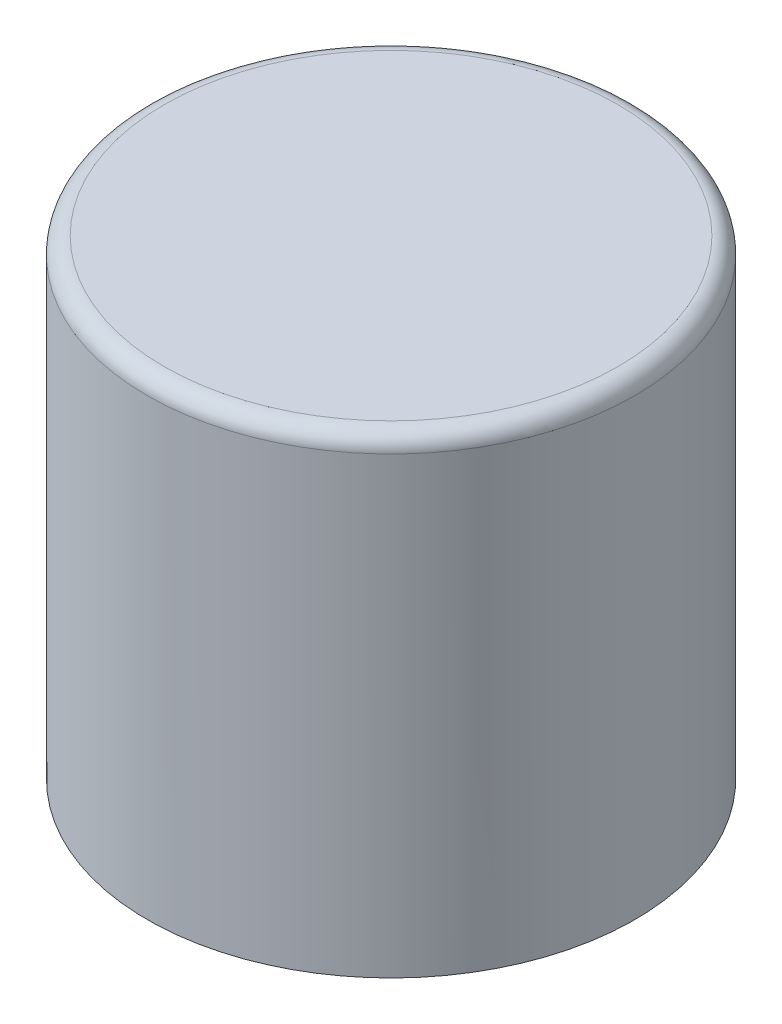
SolidWorks part; units mm, degrees
ref_plane "前视基准面" through (0, 0, 0) normal (0, 0, 1) x (1, 0, 0)
ref_plane "上视基准面" through (0, 0, 0) normal (0, 1, 0) x (1, 0, 0)
ref_plane "右视基准面" through (0, 0, 0) normal (1, 0, 0) x (0, 0, -1)
sketch "草图1" plane through (0, 0, 0) normal (0, 0, 1) x (1, 0, 0)
  line L1 (14.5, -2) -> (0, -2)
  line L2 (14.5, -2) -> (14.5, 0)
  line L3 (14.5, 0) -> (0, 0)
  line L4 (0, -2) -> (0, 0)
  line L5 (14.5, -2) -> (0, 0) construction
  line L6 (14.5, 0) -> (0, -2) construction
  line L7 (12.5, -28) -> (14.5, -28)
  line L8 (12.5, -28) -> (12.5, 0)
  line L9 (12.5, 0) -> (14.5, 0)
  line L10 (14.5, -28) -> (14.5, 0)
  line L11 (12.5, -28) -> (14.5, 0) construction
  line L12 (12.5, 0) -> (14.5, -28) construction
  point P0 (7.25, -1)
  point P5 (13.5, -14)
  dimension "D1" = 12.5
  dimension "D2" = 14.5
  dimension "D3" = 28
  dimension "D4" = 2
revolve "旋转1" add sketch "草图1" angle 360 about L4
fillet "圆角1" radius 1 1 edges at (0, 0, -14.5)
